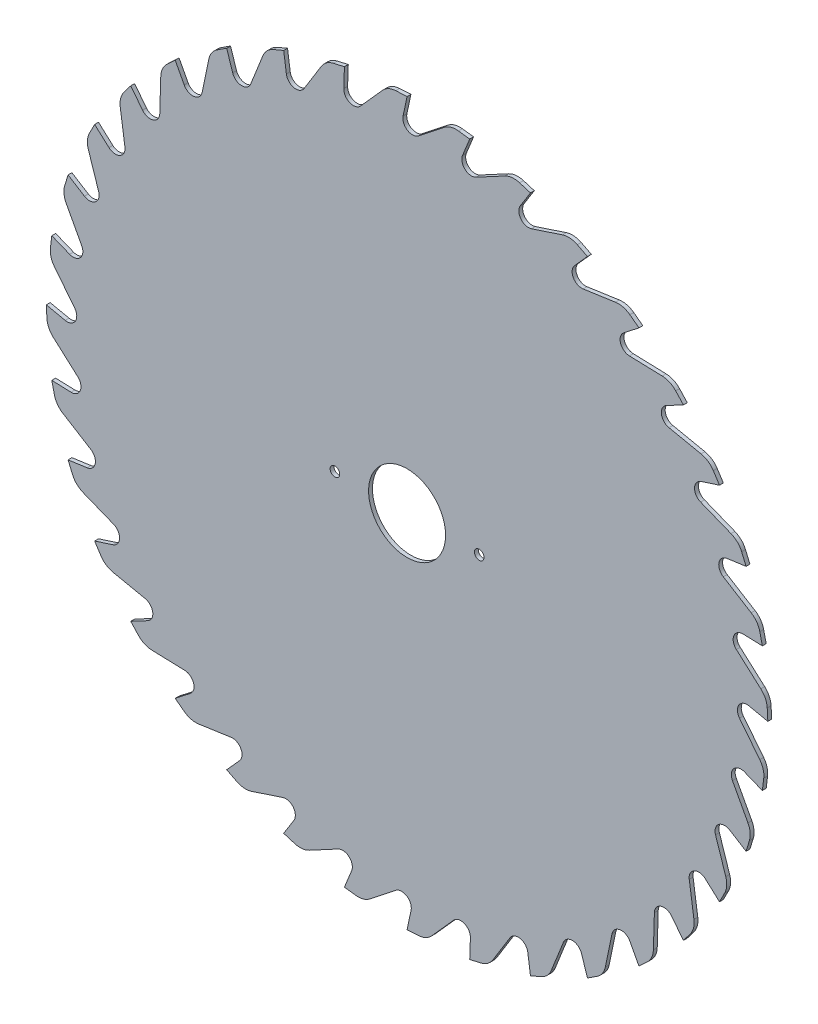
SolidWorks part; units mm, degrees
material "Nichtrostender Chromstahl"
ref_plane "Plane1" through (0, 0, 0) normal (0, 0, 1) x (1, 0, 0)
ref_plane "Plane2" through (0, 0, 0) normal (0, 1, 0) x (1, 0, 0)
ref_plane "Plane3" through (0, 0, 0) normal (1, 0, 0) x (0, 0, -1)
sketch "Sketch1" plane through (0, 0, 0) normal (0, 0, 1) x (1, 0, 0)
  line L0 (0, 375) -> (-4.1582, 355.437)
  line L1 (11.8141, 345.5047) -> (38.5722, 366.5984)
  line L2 (53.3912, 370.7428) -> (65.1181, 369.3029)
  line L3 (0, 0) -> (0, 375) construction
  line L4 (0, 0) -> (65.1181, 369.3029) construction
  line L5 (65.1181, 369.3029) -> (57.6259, 350.7592)
  line L6 (71.6308, 338.2042) -> (101.6453, 354.331)
  line L7 (116.9589, 355.8391) -> (128.2576, 352.3847)
  line L8 (128.2576, 352.3847) -> (117.6592, 335.4238)
  line L9 (129.2711, 320.6275) -> (161.63, 331.2973)
  line L10 (176.9728, 330.1234) -> (187.5, 324.7595)
  line L11 (187.5, 324.7595) -> (174.1174, 309.8966)
  line L12 (182.9836, 293.3088) -> (216.7037, 298.1974)
  line L13 (231.6095, 294.3771) -> (241.0454, 287.2667)
  line L14 (241.0454, 287.2667) -> (225.2851, 274.9534)
  line L15 (231.1362, 257.078) -> (265.1929, 256.0369)
  line L16 (279.2089, 249.6863) -> (287.2667, 241.0454)
  line L17 (287.2667, 241.0454) -> (269.6077, 231.6559)
  line L18 (272.2659, 213.036) -> (305.6244, 206.0969)
  line L19 (318.3246, 197.4088) -> (324.7595, 187.5)
  line L20 (324.7595, 187.5) -> (305.7384, 181.3197)
  line L21 (305.1228, 162.5211) -> (336.7696, 149.8947)
  line L22 (347.7683, 139.1333) -> (352.3847, 128.2576)
  line L23 (352.3847, 128.2576) -> (332.5794, 125.4741)
  line L24 (328.7088, 107.068) -> (357.6823, 89.1381)
  line L25 (366.6451, 76.6302) -> (369.3029, 65.1181)
  line L26 (369.3029, 65.1181) -> (349.3151, 65.8161)
  line L27 (342.3072, 48.3617) -> (367.7269, 25.673)
  line L28 (374.3817, 11.7987) -> (375, 0)
  line L29 (375, 0) -> (355.437, 4.1582)
  line L30 (345.5047, -11.8141) -> (366.5984, -38.5722)
  line L31 (370.7428, -53.3912) -> (369.3029, -65.1181)
  line L32 (369.3029, -65.1181) -> (350.7592, -57.6259)
  line L33 (338.2042, -71.6308) -> (354.331, -101.6453)
  line L34 (355.8391, -116.9589) -> (352.3847, -128.2576)
  line L35 (352.3847, -128.2576) -> (335.4238, -117.6592)
  line L36 (320.6275, -129.2711) -> (331.2973, -161.63)
  line L37 (330.1234, -176.9728) -> (324.7595, -187.5)
  line L38 (324.7595, -187.5) -> (309.8966, -174.1174)
  line L39 (293.3088, -182.9836) -> (298.1974, -216.7037)
  line L40 (294.3771, -231.6095) -> (287.2667, -241.0454)
  line L41 (287.2667, -241.0454) -> (274.9534, -225.2851)
  line L42 (257.078, -231.1362) -> (256.0369, -265.1929)
  line L43 (249.6863, -279.2089) -> (241.0454, -287.2667)
  line L44 (241.0454, -287.2667) -> (231.6559, -269.6077)
  line L45 (213.036, -272.2659) -> (206.0969, -305.6244)
  line L46 (197.4088, -318.3246) -> (187.5, -324.7595)
  line L47 (187.5, -324.7595) -> (181.3197, -305.7384)
  line L48 (162.5211, -305.1228) -> (149.8947, -336.7696)
  line L49 (139.1333, -347.7683) -> (128.2576, -352.3847)
  line L50 (128.2576, -352.3847) -> (125.4741, -332.5794)
  line L51 (107.068, -328.7088) -> (89.1381, -357.6823)
  line L52 (76.6302, -366.6451) -> (65.1181, -369.3029)
  line L53 (65.1181, -369.3029) -> (65.8161, -349.3151)
  line L54 (48.3617, -342.3072) -> (25.673, -367.7269)
  line L55 (11.7987, -374.3817) -> (0, -375)
  line L56 (0, -375) -> (4.1582, -355.437)
  line L57 (-11.8141, -345.5047) -> (-38.5722, -366.5984)
  line L58 (-53.3912, -370.7428) -> (-65.1181, -369.3029)
  line L59 (-65.1181, -369.3029) -> (-57.6259, -350.7592)
  line L60 (-71.6308, -338.2042) -> (-101.6453, -354.331)
  line L61 (-116.9589, -355.8391) -> (-128.2576, -352.3847)
  line L62 (-128.2576, -352.3847) -> (-117.6592, -335.4238)
  line L63 (-129.2711, -320.6275) -> (-161.63, -331.2973)
  line L64 (-176.9728, -330.1234) -> (-187.5, -324.7595)
  line L65 (-187.5, -324.7595) -> (-174.1174, -309.8966)
  line L66 (-182.9836, -293.3088) -> (-216.7037, -298.1974)
  line L67 (-231.6095, -294.3771) -> (-241.0454, -287.2667)
  line L68 (-241.0454, -287.2667) -> (-225.2851, -274.9534)
  line L69 (-231.1362, -257.078) -> (-265.1929, -256.0369)
  line L70 (-279.2089, -249.6863) -> (-287.2667, -241.0454)
  line L71 (-287.2667, -241.0454) -> (-269.6077, -231.6559)
  line L72 (-272.2659, -213.036) -> (-305.6244, -206.0969)
  line L73 (-318.3246, -197.4088) -> (-324.7595, -187.5)
  line L74 (-324.7595, -187.5) -> (-305.7384, -181.3197)
  line L75 (-305.1228, -162.5211) -> (-336.7696, -149.8947)
  line L76 (-347.7683, -139.1333) -> (-352.3847, -128.2576)
  line L77 (-352.3847, -128.2576) -> (-332.5794, -125.4741)
  line L78 (-328.7088, -107.068) -> (-357.6823, -89.1381)
  line L79 (-366.6451, -76.6302) -> (-369.3029, -65.1181)
  line L80 (-369.3029, -65.1181) -> (-349.3151, -65.8161)
  line L81 (-342.3072, -48.3617) -> (-367.7269, -25.673)
  line L82 (-374.3817, -11.7987) -> (-375, 0)
  line L83 (-375, 0) -> (-355.437, -4.1582)
  line L84 (-345.5047, 11.8141) -> (-366.5984, 38.5722)
  line L85 (-370.7428, 53.3912) -> (-369.3029, 65.1181)
  line L86 (-369.3029, 65.1181) -> (-350.7592, 57.6259)
  line L87 (-338.2042, 71.6308) -> (-354.331, 101.6453)
  line L88 (-355.8391, 116.9589) -> (-352.3847, 128.2576)
  line L89 (-352.3847, 128.2576) -> (-335.4238, 117.6592)
  line L90 (-320.6275, 129.2711) -> (-331.2973, 161.63)
  line L91 (-330.1234, 176.9728) -> (-324.7595, 187.5)
  line L92 (-324.7595, 187.5) -> (-309.8966, 174.1174)
  line L93 (-293.3088, 182.9836) -> (-298.1974, 216.7037)
  line L94 (-294.3771, 231.6095) -> (-287.2667, 241.0454)
  line L95 (-287.2667, 241.0454) -> (-274.9534, 225.2851)
  line L96 (-257.078, 231.1362) -> (-256.0369, 265.1929)
  line L97 (-249.6863, 279.2089) -> (-241.0454, 287.2667)
  line L98 (-241.0454, 287.2667) -> (-231.6559, 269.6077)
  line L99 (-213.036, 272.2659) -> (-206.0969, 305.6244)
  line L100 (-197.4088, 318.3246) -> (-187.5, 324.7595)
  line L101 (-187.5, 324.7595) -> (-181.3197, 305.7384)
  line L102 (-162.5211, 305.1228) -> (-149.8947, 336.7696)
  line L103 (-139.1333, 347.7683) -> (-128.2576, 352.3847)
  line L104 (-128.2576, 352.3847) -> (-125.4741, 332.5794)
  line L105 (-107.068, 328.7088) -> (-89.1381, 357.6823)
  line L106 (-76.6302, 366.6451) -> (-65.1181, 369.3029)
  line L107 (-65.1181, 369.3029) -> (-65.8161, 349.3151)
  line L108 (-48.3617, 342.3072) -> (-25.673, 367.7269)
  line L109 (-11.7987, 374.3817) -> (0, 375)
  line L110 (0, 375) -> (-26.9731, 375) construction
  circle A0 centre (0, 0) radius 375 construction
  arc A1 (11.8141, 345.5047) -> (-4.1582, 355.437) centre (5.6232, 353.3579) cw
  arc A2 (53.3912, 370.7428) -> (38.5722, 366.5984) centre (50.9538, 350.8919) ccw
  arc A3 (71.6308, 338.2042) -> (57.6259, 350.7592) centre (66.8978, 347.0132) cw
  arc A4 (116.9589, 355.8391) -> (101.6453, 354.331) centre (111.1114, 336.713) ccw
  arc A5 (129.2711, 320.6275) -> (117.6592, 335.4238) centre (126.1396, 330.1246) cw
  arc A6 (176.9728, 330.1234) -> (161.63, 331.2973) centre (167.893, 312.3033) ccw
  arc A7 (182.9836, 293.3088) -> (174.1174, 309.8966) centre (181.5488, 303.2053) cw
  arc A8 (231.6095, 294.3771) -> (216.7037, 298.1974) centre (219.5732, 278.4044) ccw
  arc A9 (231.1362, 257.078) -> (225.2851, 274.9534) centre (231.4418, 267.0733) cw
  arc A10 (279.2089, 249.6863) -> (265.1929, 256.0369) centre (264.5818, 236.0463) ccw
  arc A11 (272.2659, 213.036) -> (269.6077, 231.6559) centre (274.3024, 222.8264) cw
  arc A12 (318.3246, 197.4088) -> (305.6244, 206.0969) centre (301.5512, 186.5161) ccw
  arc A13 (305.1228, 162.5211) -> (305.7384, 181.3197) centre (308.8286, 171.8091) cw
  arc A14 (347.7683, 139.1333) -> (336.7696, 149.8947) centre (329.3582, 131.3186) ccw
  arc A15 (328.7088, 107.068) -> (332.5794, 125.4741) centre (333.9711, 115.5714) cw
  arc A16 (366.6451, 76.6302) -> (357.6823, 89.1381) centre (347.1577, 72.1312) ccw
  arc A17 (342.3072, 48.3617) -> (349.3151, 65.8161) centre (348.9661, 55.8221) cw
  arc A18 (374.3817, 11.7987) -> (367.7269, 25.673) centre (354.4091, 10.752) ccw
  arc A19 (345.5047, -11.8141) -> (355.437, 4.1582) centre (353.3579, -5.6232) cw
  arc A20 (370.7428, -53.3912) -> (366.5984, -38.5722) centre (350.8919, -50.9538) ccw
  arc A21 (338.2042, -71.6308) -> (350.7592, -57.6259) centre (347.0132, -66.8978) cw
  arc A22 (355.8391, -116.9589) -> (354.331, -101.6453) centre (336.713, -111.1114) ccw
  arc A23 (320.6275, -129.2711) -> (335.4238, -117.6592) centre (330.1246, -126.1396) cw
  arc A24 (330.1234, -176.9728) -> (331.2973, -161.63) centre (312.3033, -167.893) ccw
  arc A25 (293.3088, -182.9836) -> (309.8966, -174.1174) centre (303.2053, -181.5488) cw
  arc A26 (294.3771, -231.6095) -> (298.1974, -216.7037) centre (278.4044, -219.5732) ccw
  arc A27 (257.078, -231.1362) -> (274.9534, -225.2851) centre (267.0733, -231.4418) cw
  arc A28 (249.6863, -279.2089) -> (256.0369, -265.1929) centre (236.0463, -264.5818) ccw
  arc A29 (213.036, -272.2659) -> (231.6559, -269.6077) centre (222.8264, -274.3024) cw
  arc A30 (197.4088, -318.3246) -> (206.0969, -305.6244) centre (186.5161, -301.5512) ccw
  arc A31 (162.5211, -305.1228) -> (181.3197, -305.7384) centre (171.8091, -308.8286) cw
  arc A32 (139.1333, -347.7683) -> (149.8947, -336.7696) centre (131.3186, -329.3582) ccw
  arc A33 (107.068, -328.7088) -> (125.4741, -332.5794) centre (115.5714, -333.9711) cw
  arc A34 (76.6302, -366.6451) -> (89.1381, -357.6823) centre (72.1312, -347.1577) ccw
  arc A35 (48.3617, -342.3072) -> (65.8161, -349.3151) centre (55.8221, -348.9661) cw
  arc A36 (11.7987, -374.3817) -> (25.673, -367.7269) centre (10.752, -354.4091) ccw
  arc A37 (-11.8141, -345.5047) -> (4.1582, -355.437) centre (-5.6232, -353.3579) cw
  arc A38 (-53.3912, -370.7428) -> (-38.5722, -366.5984) centre (-50.9538, -350.8919) ccw
  arc A39 (-71.6308, -338.2042) -> (-57.6259, -350.7592) centre (-66.8978, -347.0132) cw
  arc A40 (-116.9589, -355.8391) -> (-101.6453, -354.331) centre (-111.1114, -336.713) ccw
  arc A41 (-129.2711, -320.6275) -> (-117.6592, -335.4238) centre (-126.1396, -330.1246) cw
  arc A42 (-176.9728, -330.1234) -> (-161.63, -331.2973) centre (-167.893, -312.3033) ccw
  arc A43 (-182.9836, -293.3088) -> (-174.1174, -309.8966) centre (-181.5488, -303.2053) cw
  arc A44 (-231.6095, -294.3771) -> (-216.7037, -298.1974) centre (-219.5732, -278.4044) ccw
  arc A45 (-231.1362, -257.078) -> (-225.2851, -274.9534) centre (-231.4418, -267.0733) cw
  arc A46 (-279.2089, -249.6863) -> (-265.1929, -256.0369) centre (-264.5818, -236.0463) ccw
  arc A47 (-272.2659, -213.036) -> (-269.6077, -231.6559) centre (-274.3024, -222.8264) cw
  arc A48 (-318.3246, -197.4088) -> (-305.6244, -206.0969) centre (-301.5512, -186.5161) ccw
  arc A49 (-305.1228, -162.5211) -> (-305.7384, -181.3197) centre (-308.8286, -171.8091) cw
  arc A50 (-347.7683, -139.1333) -> (-336.7696, -149.8947) centre (-329.3582, -131.3186) ccw
  arc A51 (-328.7088, -107.068) -> (-332.5794, -125.4741) centre (-333.9711, -115.5714) cw
  arc A52 (-366.6451, -76.6302) -> (-357.6823, -89.1381) centre (-347.1577, -72.1312) ccw
  arc A53 (-342.3072, -48.3617) -> (-349.3151, -65.8161) centre (-348.9661, -55.8221) cw
  arc A54 (-374.3817, -11.7987) -> (-367.7269, -25.673) centre (-354.4091, -10.752) ccw
  arc A55 (-345.5047, 11.8141) -> (-355.437, -4.1582) centre (-353.3579, 5.6232) cw
  arc A56 (-370.7428, 53.3912) -> (-366.5984, 38.5722) centre (-350.8919, 50.9538) ccw
  arc A57 (-338.2042, 71.6308) -> (-350.7592, 57.6259) centre (-347.0132, 66.8978) cw
  arc A58 (-355.8391, 116.9589) -> (-354.331, 101.6453) centre (-336.713, 111.1114) ccw
  arc A59 (-320.6275, 129.2711) -> (-335.4238, 117.6592) centre (-330.1246, 126.1396) cw
  arc A60 (-330.1234, 176.9728) -> (-331.2973, 161.63) centre (-312.3033, 167.893) ccw
  arc A61 (-293.3088, 182.9836) -> (-309.8966, 174.1174) centre (-303.2053, 181.5488) cw
  arc A62 (-294.3771, 231.6095) -> (-298.1974, 216.7037) centre (-278.4044, 219.5732) ccw
  arc A63 (-257.078, 231.1362) -> (-274.9534, 225.2851) centre (-267.0733, 231.4418) cw
  arc A64 (-249.6863, 279.2089) -> (-256.0369, 265.1929) centre (-236.0463, 264.5818) ccw
  arc A65 (-213.036, 272.2659) -> (-231.6559, 269.6077) centre (-222.8264, 274.3024) cw
  arc A66 (-197.4088, 318.3246) -> (-206.0969, 305.6244) centre (-186.5161, 301.5512) ccw
  arc A67 (-162.5211, 305.1228) -> (-181.3197, 305.7384) centre (-171.8091, 308.8286) cw
  arc A68 (-139.1333, 347.7683) -> (-149.8947, 336.7696) centre (-131.3186, 329.3582) ccw
  arc A69 (-107.068, 328.7088) -> (-125.4741, 332.5794) centre (-115.5714, 333.9711) cw
  arc A70 (-76.6302, 366.6451) -> (-89.1381, 357.6823) centre (-72.1312, 347.1577) ccw
  arc A71 (-48.3617, 342.3072) -> (-65.8161, 349.3151) centre (-55.8221, 348.9661) cw
  arc A72 (-11.7987, 374.3817) -> (-25.673, 367.7269) centre (-10.752, 354.4091) ccw
  point P10 (45.1181, 371.7586)
extrude "Dicke" add sketch "Sketch1" along normal blind 4
sketch "Sketch2" plane through (0, 0, 4) normal (0, 0, 1) x (1, 0, 0)
  line L0 (-102.6303, 0) -> (96.0016, 0) construction
  circle A0 centre (0, 0) radius 75 construction
  circle A1 centre (75, 0) radius 5
  circle A2 centre (-75, 0) radius 5
  circle A3 centre (0, 0) radius 40
  dimension "Durchmesser Zentrumbohrung" = 80
  dimension "TK Mitnehmerbohrungen" = 150
  dimension "Durchmesser mitnehmerbohrungen" = 10
extrude "Linear Cut Extrude1" cut sketch "Sketch2" against normal through all
equation "\"D6@Sketch1\" = 2 * \"Zahnwinkelversatz@Sketch1\""
equation "\"D4@Sketch1\" = 2 * \"Zahnwinkelversatz@Sketch1\""
equation "\"D3@Sketch1\" = \"Zahnwinkelversatz@Sketch1\""
equation "\"D8@Sketch1\" = 2*\"Zahnwinkelversatz@Sketch1\""
